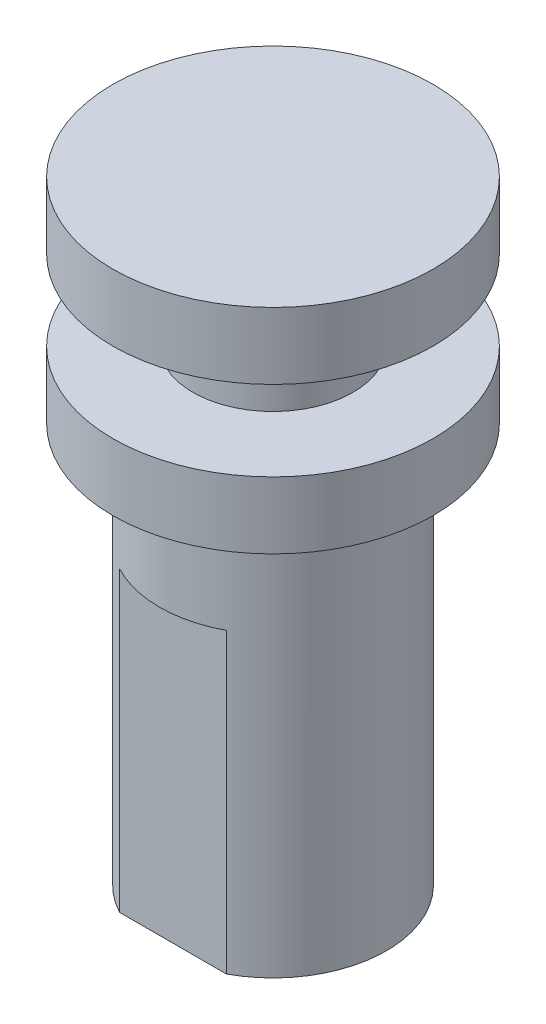
from build123d import *

# Parameters (mm, degrees)
SKETCH1_R             = 3
BOSS_EXTRUDE1_DEPTH   = 3
SKETCH2_R             = 6
BOSS_EXTRUDE2_DEPTH   = 2.5
BOSS_EXTRUDE3_START   = 2.5
SKETCH3_R             = 6
BOSS_EXTRUDE3_DEPTH   = 2.5
SKETCH4_R             = 4.25
BOSS_EXTRUDE4_DEPTH   = 15
SKETCH5_R             = 1
CUT_EXTRUDE1_DEPTH    = 7
M5_TAPPED_HOLE1_D     = 4.2
M5_TAPPED_HOLE1_DEPTH = 12
M5_TAPPED_HOLE1_TIP   = 1.2618073
SKETCH7_W             = 2.207825045
SKETCH7_H             = 11.152764798
CUT_EXTRUDE2_DEPTH    = 5


with BuildPart() as part:
    # Sketch1 → Boss-Extrude1 (new body)
    with BuildSketch(Plane(origin=(0, 0, 0), x_dir=(1, 0, 0), z_dir=(0, 1, 0))):
        with Locations(Location((0, 0, 0), (0, 0, 270))):
            Circle(SKETCH1_R)
    extrude(amount=BOSS_EXTRUDE1_DEPTH)

    # Sketch2 → Boss-Extrude2 (add)
    with BuildSketch(Plane(origin=(0, 3, 0), x_dir=(1, 0, 0), z_dir=(0, 1, 0))):
        with Locations(Location((0, 0, 0), (0, 0, 270))):
            Circle(SKETCH2_R)
    extrude(amount=BOSS_EXTRUDE2_DEPTH)

    # Sketch3 → Boss-Extrude3 (add)
    with BuildSketch(Plane.XZ.offset(BOSS_EXTRUDE3_START)):
        with Locations(Location((0, 0, 0), (0, 0, 90))):
            Circle(SKETCH3_R)
    extrude(amount=-BOSS_EXTRUDE3_DEPTH)

    # Sketch4 → Boss-Extrude4 (add)
    with BuildSketch(Plane.XZ.offset(2.5)):
        with Locations(Location((0, 0, 0), (0, 0, 270))):
            Circle(SKETCH4_R)
    extrude(amount=BOSS_EXTRUDE4_DEPTH)

    # Sketch5 → Cut-Extrude1 (cut)
    with BuildSketch(Plane.XZ.offset(17.5)):
        with Locations(Location((0, 0, 0), (0, 0, 270))):
            Circle(SKETCH5_R)
    extrude(amount=-CUT_EXTRUDE1_DEPTH, mode=Mode.SUBTRACT)

    # M5 Tapped Hole1
    with Locations(Plane(origin=(0, -17.5, 0), x_dir=(0, 0, -1), z_dir=(0, -1, 0))):
        with Locations((0, 0)):
            Hole(M5_TAPPED_HOLE1_D / 2, depth=M5_TAPPED_HOLE1_DEPTH)
            with Locations((0, 0, -(M5_TAPPED_HOLE1_DEPTH + M5_TAPPED_HOLE1_TIP / 2))):  # 118° drill point
                Cone(0, M5_TAPPED_HOLE1_D / 2, M5_TAPPED_HOLE1_TIP, mode=Mode.SUBTRACT)

    # Sketch7 → Cut-Extrude2 (cut, symmetric)
    with BuildSketch(Plane(origin=(0, 0, 0), x_dir=(0, 0, -1), z_dir=(1, 0, 0))):
        with Locations((4.853912523, -11.923617601)):
            Rectangle(SKETCH7_W, SKETCH7_H)
        with Locations((-4.853912523, -11.923617601)):
            Rectangle(SKETCH7_W, SKETCH7_H)
    extrude(amount=CUT_EXTRUDE2_DEPTH, both=True, mode=Mode.SUBTRACT)


solid = part.part
